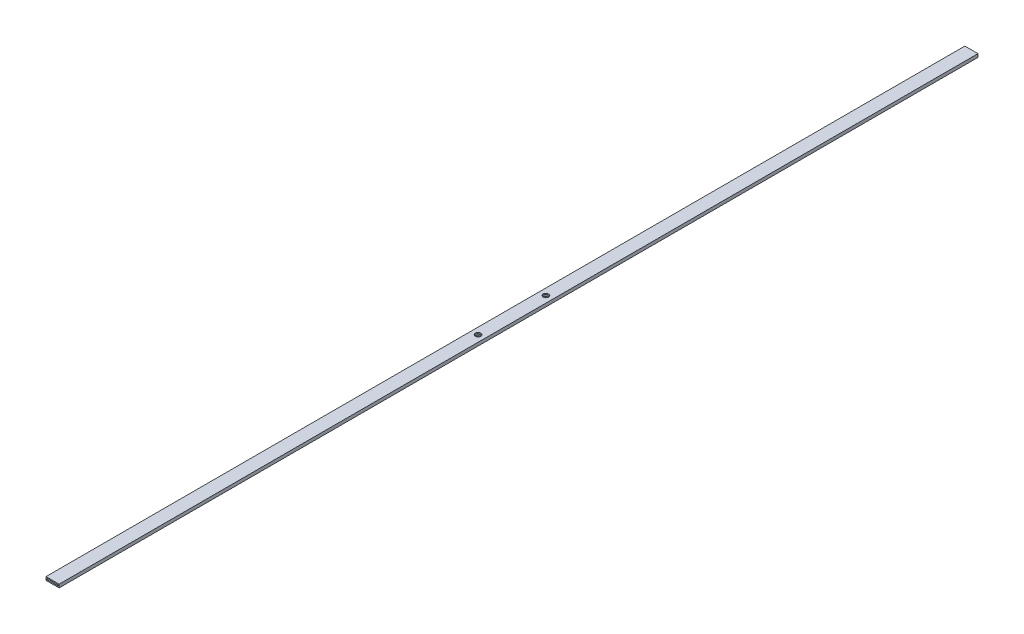
SolidWorks part; units mm, degrees
ref_plane "Front Plane" through (0, 0, 0) normal (0, 0, 1) x (1, 0, 0)
ref_plane "Top Plane" through (0, 0, 0) normal (0, 1, 0) x (1, 0, 0)
ref_plane "Right Plane" through (0, 0, 0) normal (1, 0, 0) x (0, 0, -1)
other "Configuration Table"
sketch "Sketch1" plane through (0, 0, 0) normal (0, 0, 1) x (1, 0, 0)
  line L0 (-31.901, 24.1249) -> (-19.901, 24.1249)
  line L1 (-19.901, 24.1249) -> (-19.901, 21.1249)
  line L2 (-19.901, 21.1249) -> (-31.901, 21.1249)
  line L3 (-31.901, 21.1249) -> (-31.901, 24.1249)
  dimension "D1" = 12
  dimension "D2" = 3
extrude "Boss-Extrude1" add sketch "Sketch1" along normal blind 840
sketch "Sketch2" plane through (0, 0, 840) normal (0, 0, 1) x (1, 0, 0)
  line L0 (-30.901, 23.1249) -> (-20.901, 23.1249)
  line L1 (-20.901, 23.1249) -> (-20.901, 22.1249)
  line L2 (-20.901, 22.1249) -> (-30.901, 22.1249)
  line L3 (-30.901, 22.1249) -> (-30.901, 23.1249)
  line L4 (-19.901, 24.1249) -> (-31.901, 24.1249) construction
  line L5 (-19.901, 21.1249) -> (-19.901, 24.1249) construction
  line L6 (-31.901, 21.1249) -> (-19.901, 21.1249) construction
  line L7 (-31.901, 24.1249) -> (-31.901, 21.1249) construction
  dimension "D1" = 1
  dimension "D2" = 1
  dimension "D3" = 1
  dimension "D4" = 1
extrude "Cut-Extrude1" cut sketch "Sketch2" against normal through all
sketch "Sketch3" plane through (0, 24.1249, 0) normal (0, 1, 0) x (1, 0, 0)
  line L0 (-19.901, -420) -> (-31.901, -420) construction
  line L1 (-19.901, -840) -> (-19.901, 0) construction
  line L2 (-31.901, -840) -> (-31.901, 0) construction
  line L3 (-25.901, -420) -> (-25.901, -389)
  line L4 (-25.901, -389) -> (-25.901, -451)
hole_wizard "M6 Tapped Hole1" positions "3DSketch1" profile "Sketch4" tap size "M6" standard "GB"
sketch3d "3DSketch1"
  point P0 (-25.901, 24.1249, 389)
  point P3 (-25.901, 24.1249, 451)
sketch "Sketch4" plane through (-25.901, 24.1249, 389) normal (1, 0, 0) x (0, 0, 1)
  line L0 (0, 0) -> (0, 16.5022)
  line L1 (0, 16.5022) -> (2.5, 15)
  line L2 (2.5, 15) -> (2.5, 0)
  line L5 (2.5, 0) -> (0, 0)
  line L10 (0, 16.5022) -> (-2.5, 15) construction
  line L11 (0, -6.35) -> (0, 107.95) construction
  dimension "螺纹孔钻头直径" = 5
  dimension "螺纹孔钻头深度" = 15
  dimension "导头角度" = 118
cosmetic thread "Hole thread line1" parameters "D1"=12, "D2"=6
cosmetic thread "Hole thread line2" parameters "D1"=12, "D2"=6
